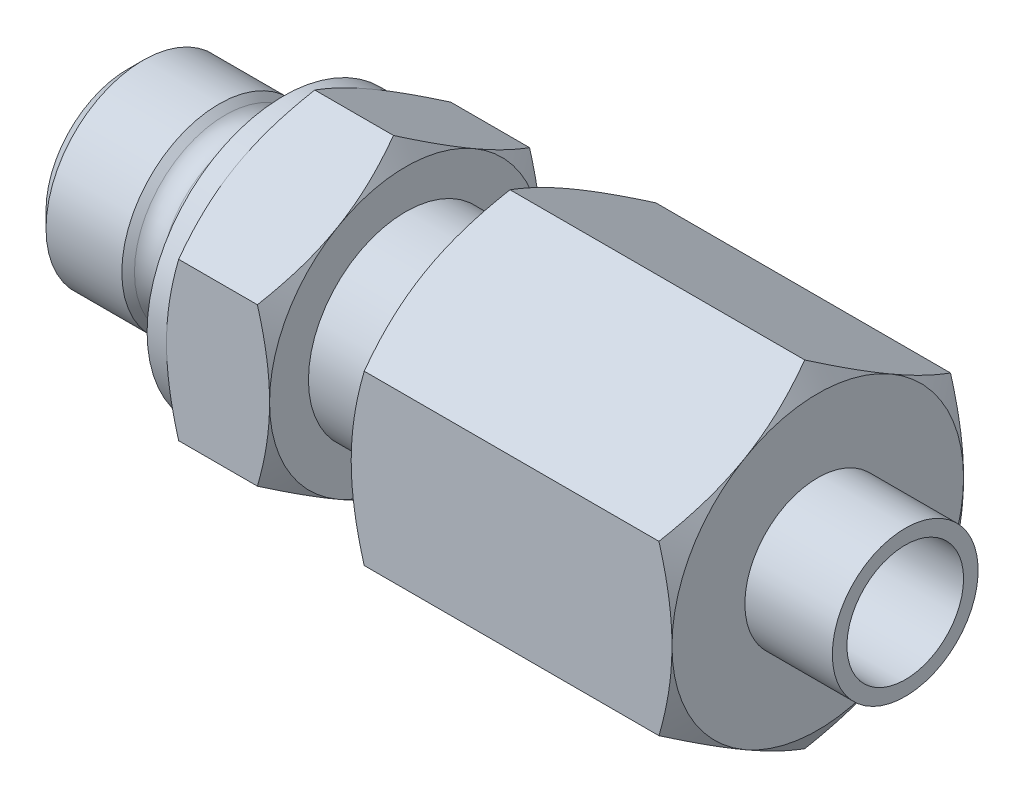
from build123d import *

# Parameters (mm, degrees)
EXTRUDE_START       = -16.5
SKETCH_3_R          = 2
EXTRUDE_2_DEPTH     = 16.5
EXTRUDE_START_2     = -5.3
SKETCH_2_R          = 2
EXTRUDE_1_DEPTH     = 5.3
SKETCH_6_R          = 3
CUT_EXTRUDE_1_DEPTH = 10


with BuildPart() as part:
    # 草图1 → 旋转1 (revolve)
    with BuildSketch(Plane.XY, mode=Mode.PRIVATE) as revolve_1_sk:
        with BuildLine():
            Line((0, 2), (0, 4.2))
            Line((0, 4.2), (0.8, 5))
            Line((0.8, 5), (4.7, 5))
            Line((4.7, 5), (5.025001538, 4.674998462))
            ThreePointArc((5.025001538, 4.674998462), (5.539435688, 4.40084215), (6.119340804, 4.460123138))
            Line((6.119340804, 4.460123138), (8, 5.25))
            Line((8, 5.25), (8, 7))
            Line((8, 7), (9, 7))
            Line((9, 7), (14.3, 7))
            Line((14.3, 7), (14.3, 5))
            Line((14.3, 5), (19, 5))
            Line((19, 5), (19, 7.5))
            Line((19, 7.5), (35.5, 7.5))
            Line((35.5, 7.5), (35.5, 3.75))
            Line((35.5, 3.75), (40, 3.75))
            Line((40, 3.75), (40, 2))
            Line((40, 2), (0, 2))
        make_face()
    revolve(revolve_1_sk.sketch.rotate(Axis((0, 0, 0), (1, 0, 0)), 90), axis=Axis((0, 0, 0), (1, 0, 0)))

    # 草图3 → 拉伸2 (add)
    with BuildSketch(Plane(origin=(35.5, 0, 0), x_dir=(0, 0, -1), z_dir=(1, 0, 0)).offset(EXTRUDE_START)):
        Polygon((7.5, -4.330127019), (7.5, 4.330127019), (0, 8.660254038), (-7.5, 4.330127019), (-7.5, -4.330127019), (0, -8.660254038), align=None)
        with Locations(Location((0, 0, 0), (0, 0, 180))):
            Circle(SKETCH_3_R, mode=Mode.SUBTRACT)
    extrude(amount=EXTRUDE_2_DEPTH)

    # 草图2 → 凸台-拉伸1 (add)
    with BuildSketch(Plane(origin=(14.3, 0, 0), x_dir=(0, 0, -1), z_dir=(1, 0, 0)).offset(EXTRUDE_START_2)):
        Polygon((-7, 4.041451884), (-7, -4.041451884), (0, -8.082903769), (7, -4.041451884), (7, 4.041451884), (0, 8.082903769), align=None)
        with Locations(Location((0, 0, 0), (0, 0, 180))):
            Circle(SKETCH_2_R, mode=Mode.SUBTRACT)
    extrude(amount=EXTRUDE_1_DEPTH)

    # 草图4 → 切除-旋转1 (revolve, cut)
    with BuildSketch(Plane.XY):
        Polygon((9, 7), (9.625214782, 8.082903769), (9, 8.082903769), align=None)
        Polygon((14.3, 7), (13.674785218, 8.082903769), (14.3, 8.082903769), align=None)
        Polygon((19, 7.5), (19.669872981, 8.660254038), (19, 8.660254038), align=None)
        Polygon((35.5, 7.5), (34.830127019, 8.660254038), (35.5, 8.660254038), align=None)
    revolve(axis=Axis((0, 0, 0), (1, 0, 0)), mode=Mode.SUBTRACT)

    # 草图6 → 切除-拉伸1 (cut)
    with BuildSketch(Plane(origin=(40, 0, 0), x_dir=(0, 0, -1), z_dir=(1, 0, 0))):
        Circle(SKETCH_6_R)
    extrude(amount=-CUT_EXTRUDE_1_DEPTH, mode=Mode.SUBTRACT)


solid = part.part
